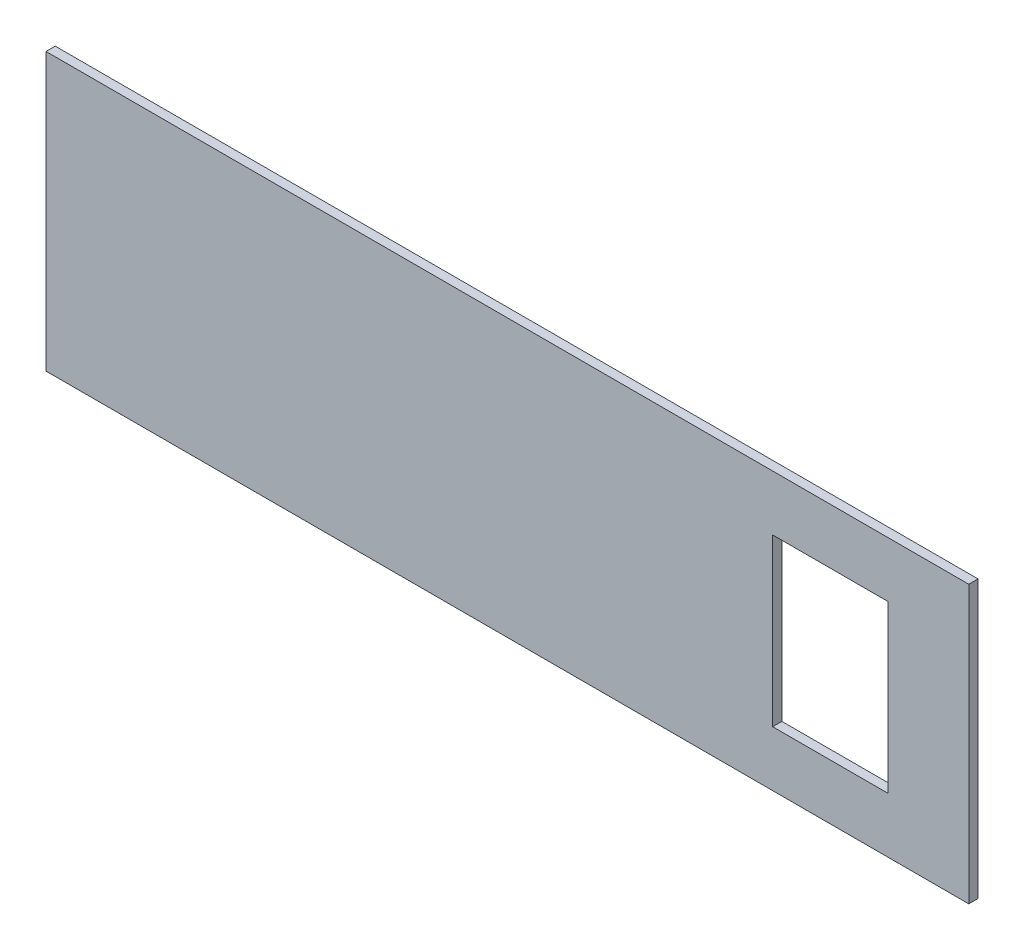
SolidWorks part; units mm, degrees
ref_plane "Front Plane" through (0, 0, 0) normal (0, 0, 1) x (1, 0, 0)
ref_plane "Top Plane" through (0, 0, 0) normal (0, 1, 0) x (1, 0, 0)
ref_plane "Right Plane" through (0, 0, 0) normal (1, 0, 0) x (0, 0, -1)
sketch "Sketch1" plane through (0, 0, 0) normal (0, 0, 1) x (1, 0, 0)
  line L1 (-1000, 300) -> (1000, 300)
  line L2 (-1000, 300) -> (-1000, -300)
  line L3 (-1000, -300) -> (1000, -300)
  line L4 (1000, 300) -> (1000, -300)
  line L5 (-1000, 300) -> (1000, -300) construction
  line L6 (-1000, -300) -> (1000, 300) construction
  point P0 (0, 0)
  dimension "D1" = 2000
  dimension "D2" = 600
extrude "Boss-Extrude1" add sketch "Sketch1" along normal blind 20
sketch "Sketch2" plane through (0, 0, 0) normal (0, 0, -1) x (-1, 0, 0)
  line L0 (-1000, -300) -> (-1000, 300) construction
  line L1 (-575, -180) -> (-825, -180)
  line L2 (-575, -180) -> (-575, 180)
  line L3 (-575, 180) -> (-825, 180)
  line L4 (-825, -180) -> (-825, 180)
  line L5 (-575, -180) -> (-825, 180) construction
  line L6 (-575, 180) -> (-825, -180) construction
  point P0 (-700, 0)
  dimension "D1" = 250
  dimension "D2" = 360
  dimension "D3" = 300
extrude "Cut-Extrude1" cut sketch "Sketch2" against normal through all
sketch "Sketch3" plane through (0, 0, 0) normal (0, 0, -1) x (-1, 0, 0)
  line L1 (-320, -47.5) -> (-380, -47.5)
  line L2 (-320, -47.5) -> (-320, 2.5)
  line L3 (-320, 2.5) -> (-380, 2.5)
  line L4 (-380, -47.5) -> (-380, 2.5)
  line L5 (-320, -47.5) -> (-380, 2.5) construction
  line L6 (-320, 2.5) -> (-380, -47.5) construction
  point P0 (-350, -22.5)
  dimension "D1" = 50
  dimension "D2" = 60
  dimension "D3" = 380
extrude "Boss-Extrude2" add sketch "Sketch3" along normal blind 51
sketch "Sketch4" plane through (0, 0, -51) normal (0, 0, -1) x (-1, 0, 0)
  line L0 (-380, 2.5) -> (-380, -47.5) construction
  line L1 (-380, -17.5) -> (-320, -17.5)
  line L2 (-380, -17.5) -> (-380, -29.5)
  line L3 (-380, -29.5) -> (-320, -29.5)
  line L4 (-320, -17.5) -> (-320, -29.5)
  line L5 (-320, -47.5) -> (-320, 2.5) construction
  line L7 (-320, 2.5) -> (-380, 2.5) construction
  dimension "D1" = 12
  dimension "D2" = 20
extrude "Cut-Extrude2" cut sketch "Sketch4" against normal blind 40
fillet "Fillet1" radius 12 4 edges at (320, -38.5, -51) (320, -7.5, -51) (380, -7.5, -51) (380, -38.5, -51)
sketch "Sketch5" plane through (0, -47.5, 0) normal (0, -1, 0) x (1, 0, 0)
  line L0 (350, -51) -> (350, -6.9413) construction
  line L1 (368, -51) -> (332, -51) construction
  circle A0 centre (350, -26) radius 10
  dimension "D1" = 20
  dimension "D2" = 25
extrude "Cut-Extrude3" cut sketch "Sketch5" against normal through all
pattern_linear "LPattern1" count 2 spacing 120 along (-1, 0, 0) of "Boss-Extrude2", "Cut-Extrude3", "Fillet1", "Cut-Extrude2"
